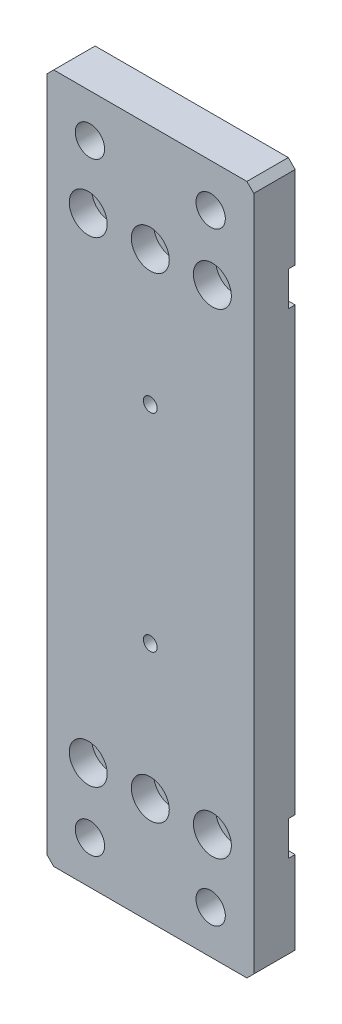
from build123d import *

# Parameters (mm, degrees)
SKETCH1_W                                            = 60
SKETCH1_H                                            = 200
BOSS_EXTRUDE1_DEPTH                                  = 6
CHAMFER1_SIZE                                        = 2
SKETCH2_W                                            = 60
SKETCH2_H                                            = 10
CUT_EXTRUDE1_DEPTH                                   = 2
HOLE_SIZE_PER_SOCKET_HEAD_CAP_SCREW_TYPE_D           = 6.5
HOLE_SIZE_PER_SOCKET_HEAD_CAP_SCREW_TYPE_CBORE_D     = 11
HOLE_SIZE_PER_SOCKET_HEAD_CAP_SCREW_TYPE_CBORE_DEPTH = 6.5
SKETCH5_R                                            = 4.25
CUT_EXTRUDE2_DEPTH                                   = 106.090437243
SKETCH6_R                                            = 2
CUT_EXTRUDE3_DEPTH                                   = 106.090437243


with BuildPart() as part:
    # Sketch1 → Boss-Extrude1 (new, symmetric)
    with BuildSketch(Plane.XY):
        Rectangle(SKETCH1_W, SKETCH1_H)
    extrude(amount=BOSS_EXTRUDE1_DEPTH, both=True)

    # Chamfer1
    chamfer1_edges = [part.edges().sort_by_distance(p)[0] for p in [
        (30, -100, 0),
        (-30, -100, 0),
        (-30, 100, 0),
        (30, 100, 0),
    ]]
    chamfer(chamfer1_edges, length=CHAMFER1_SIZE)

    # Sketch2 → Cut-Extrude1 (cut)
    with BuildSketch(Plane(origin=(0, 0, -6), x_dir=(-1, 0, 0), z_dir=(0, 0, -1))):
        with Locations((0, 69)):
            Rectangle(SKETCH2_W, SKETCH2_H)
        with Locations((0, -69)):
            Rectangle(SKETCH2_W, SKETCH2_H)
    extrude(amount=-CUT_EXTRUDE1_DEPTH, mode=Mode.SUBTRACT)

    # Hole size per socket head cap screw type 1 (through all)
    with Locations(Plane.XY.offset(6)):
        with Locations((-18, -69), (0, -69), (18, -69), (18, 69), (0, 69), (-18, 69)):
            CounterBoreHole(HOLE_SIZE_PER_SOCKET_HEAD_CAP_SCREW_TYPE_D / 2, HOLE_SIZE_PER_SOCKET_HEAD_CAP_SCREW_TYPE_CBORE_D / 2, HOLE_SIZE_PER_SOCKET_HEAD_CAP_SCREW_TYPE_CBORE_DEPTH)

    # Sketch5 → Cut-Extrude2 (cut, through all)
    with BuildSketch(Plane(origin=(0, 0, -6), x_dir=(-1, 0, 0), z_dir=(0, 0, -1))):
        with Locations((17.5, 87.5)):
            Circle(SKETCH5_R)
        with Locations((-17.5, 87.5)):
            Circle(SKETCH5_R)
        with Locations((17.5, -87.5)):
            Circle(SKETCH5_R)
        with Locations((-17.5, -87.5)):
            Circle(SKETCH5_R)
    extrude(amount=-CUT_EXTRUDE2_DEPTH, mode=Mode.SUBTRACT)

    # Sketch6 → Cut-Extrude3 (cut, through all)
    with BuildSketch(Plane.XY.offset(6)):
        with Locations((0, 30)):
            Circle(SKETCH6_R)
        with Locations((0, -30)):
            Circle(SKETCH6_R)
    extrude(amount=-CUT_EXTRUDE3_DEPTH, mode=Mode.SUBTRACT)


solid = part.part
